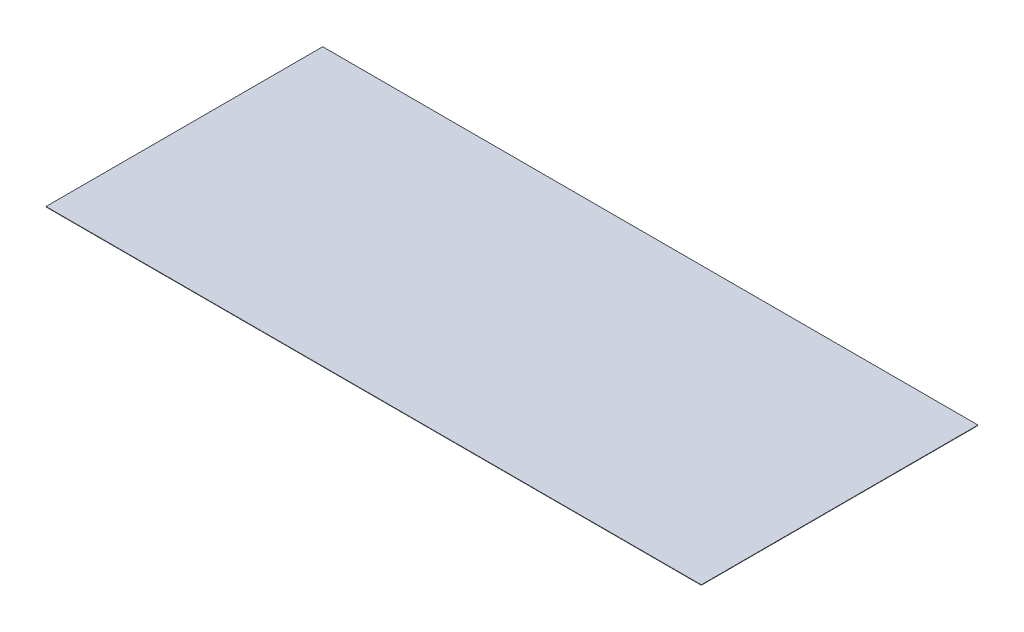
SolidWorks part; units mm, degrees
ref_plane "Front Plane" through (0, 0, 0) normal (0, 0, 1) x (1, 0, 0)
ref_plane "Top Plane" through (0, 0, 0) normal (0, 1, 0) x (1, 0, 0)
ref_plane "Right Plane" through (0, 0, 0) normal (1, 0, 0) x (0, 0, -1)
sketch "Sketch 1" plane through (0, 0, 0) normal (0, 1, 0) x (1, 0, 0)
  line L1 (-2510, -1060) -> (2510, -1060)
  line L2 (-2510, -1060) -> (-2510, 1060)
  line L3 (-2510, 1060) -> (2510, 1060)
  line L4 (2510, -1060) -> (2510, 1060)
  line L5 (-2510, -1060) -> (2510, 1060) construction
  line L6 (-2510, 1060) -> (2510, -1060) construction
  point P0 (0, 0)
  dimension "D1" = 5020
  dimension "D2" = 2120
extrude "Boss-Extrude 1" add sketch "Sketch 1" along normal blind 3
